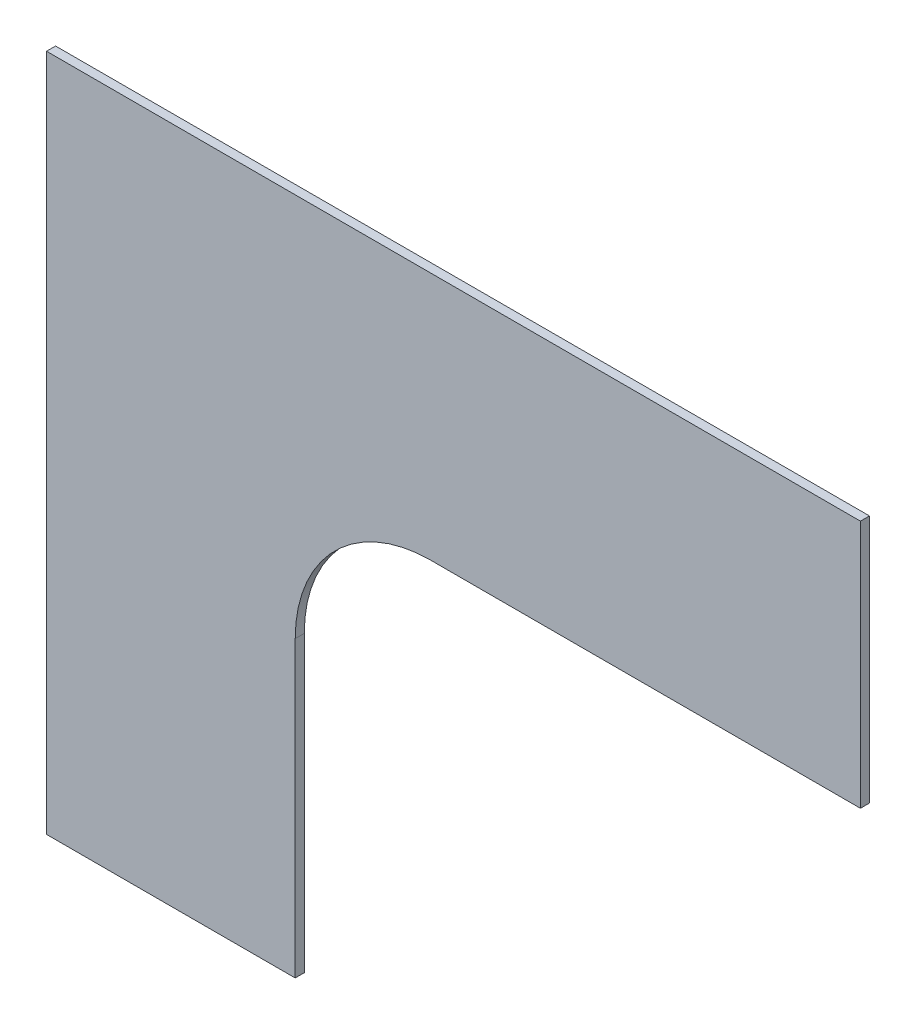
SolidWorks part; units mm, degrees
material "轻木"
ref_plane "Front Plane" through (0, 0, 0) normal (0, 0, 1) x (1, 0, 0)
ref_plane "Top Plane" through (0, 0, 0) normal (0, 1, 0) x (1, 0, 0)
ref_plane "Right Plane" through (0, 0, 0) normal (1, 0, 0) x (0, 0, -1)
sketch "Sketch1" plane through (0, 0, 0) normal (0, 0, 1) x (1, 0, 0)
  line L0 (0, 0) -> (0, 1500)
  line L1 (0, 1500) -> (1800, 1500)
  line L2 (1800, 1500) -> (1800, 950)
  line L3 (1800, 950) -> (850, 950)
  line L4 (550, 650) -> (550, 0)
  line L5 (550, 0) -> (0, 0)
  arc A0 (850, 950) -> (550, 650) centre (850, 650) ccw
  dimension "D5" = 300
  dimension "D1" = 1800
  dimension "D2" = 1500
  dimension "D3" = 550
  dimension "D4" = 550
extrude "Boss-Extrude1" add sketch "Sketch1" along normal blind 20
